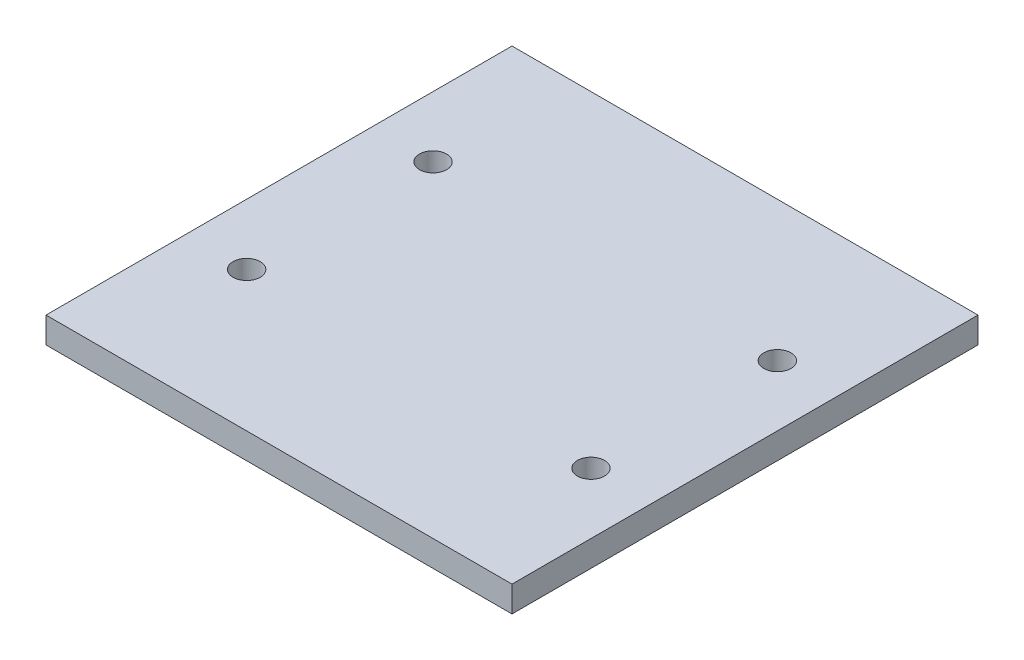
SolidWorks part; units mm, degrees
material "普通碳钢"
ref_plane "Front Plane" through (0, 0, 0) normal (0, 0, 1) x (1, 0, 0)
ref_plane "Top Plane" through (0, 0, 0) normal (0, 1, 0) x (1, 0, 0)
ref_plane "Right Plane" through (0, 0, 0) normal (1, 0, 0) x (0, 0, -1)
sketch "Sketch1" plane through (0, 0, 0) normal (0, 1, 0) x (1, 0, 0)
  line L1 (-180, 180) -> (-180, -180)
  line L2 (-180, -180) -> (180, -180)
  line L3 (180, -180) -> (180, 180)
  line L4 (180, 180) -> (-180, 180)
  point P0 (0, 180)
  point P1 (-180, 0)
  dimension "D1" = 360
  dimension "D2" = 360
extrude "Extrude1" add sketch "Sketch1" along normal mid plane 20
hole_wizard "M24 Tapped Hole1" positions "Sketch3" profile "Sketch2" tap size "M24" standard "GB" end condition through all
sketch "Sketch3" plane through (0, 10, 0) normal (0, 1, 0) x (-1, 0, 0)
  line L1 (180, -180) -> (180, 180) construction
  point P0 (133, -72)
  dimension "D1" = 47
  dimension "D2" = 72
sketch "Sketch2" plane through (-133, 10, -72) normal (1, 0, 0) x (0, 0, 1)
  line L0 (0, 0) -> (0, 20)
  line L1 (0, 20) -> (10.5, 20)
  line L2 (10.5, 20) -> (10.5, 0)
  line L5 (10.5, 0) -> (0, 0)
  line L11 (0, -6.35) -> (0, 107.95) construction
  dimension "通孔螺纹孔钻头直径" = 21
  dimension "通孔螺纹孔钻头深度" = 20
cosmetic thread "Hole cosmetic thread1" parameters "D2"=24
pattern_linear "LPattern2" count 2 spacing 144 along (0, 0, 1) count 2 spacing 266 along (1, 0, 0) of "M24 Tapped Hole1"
